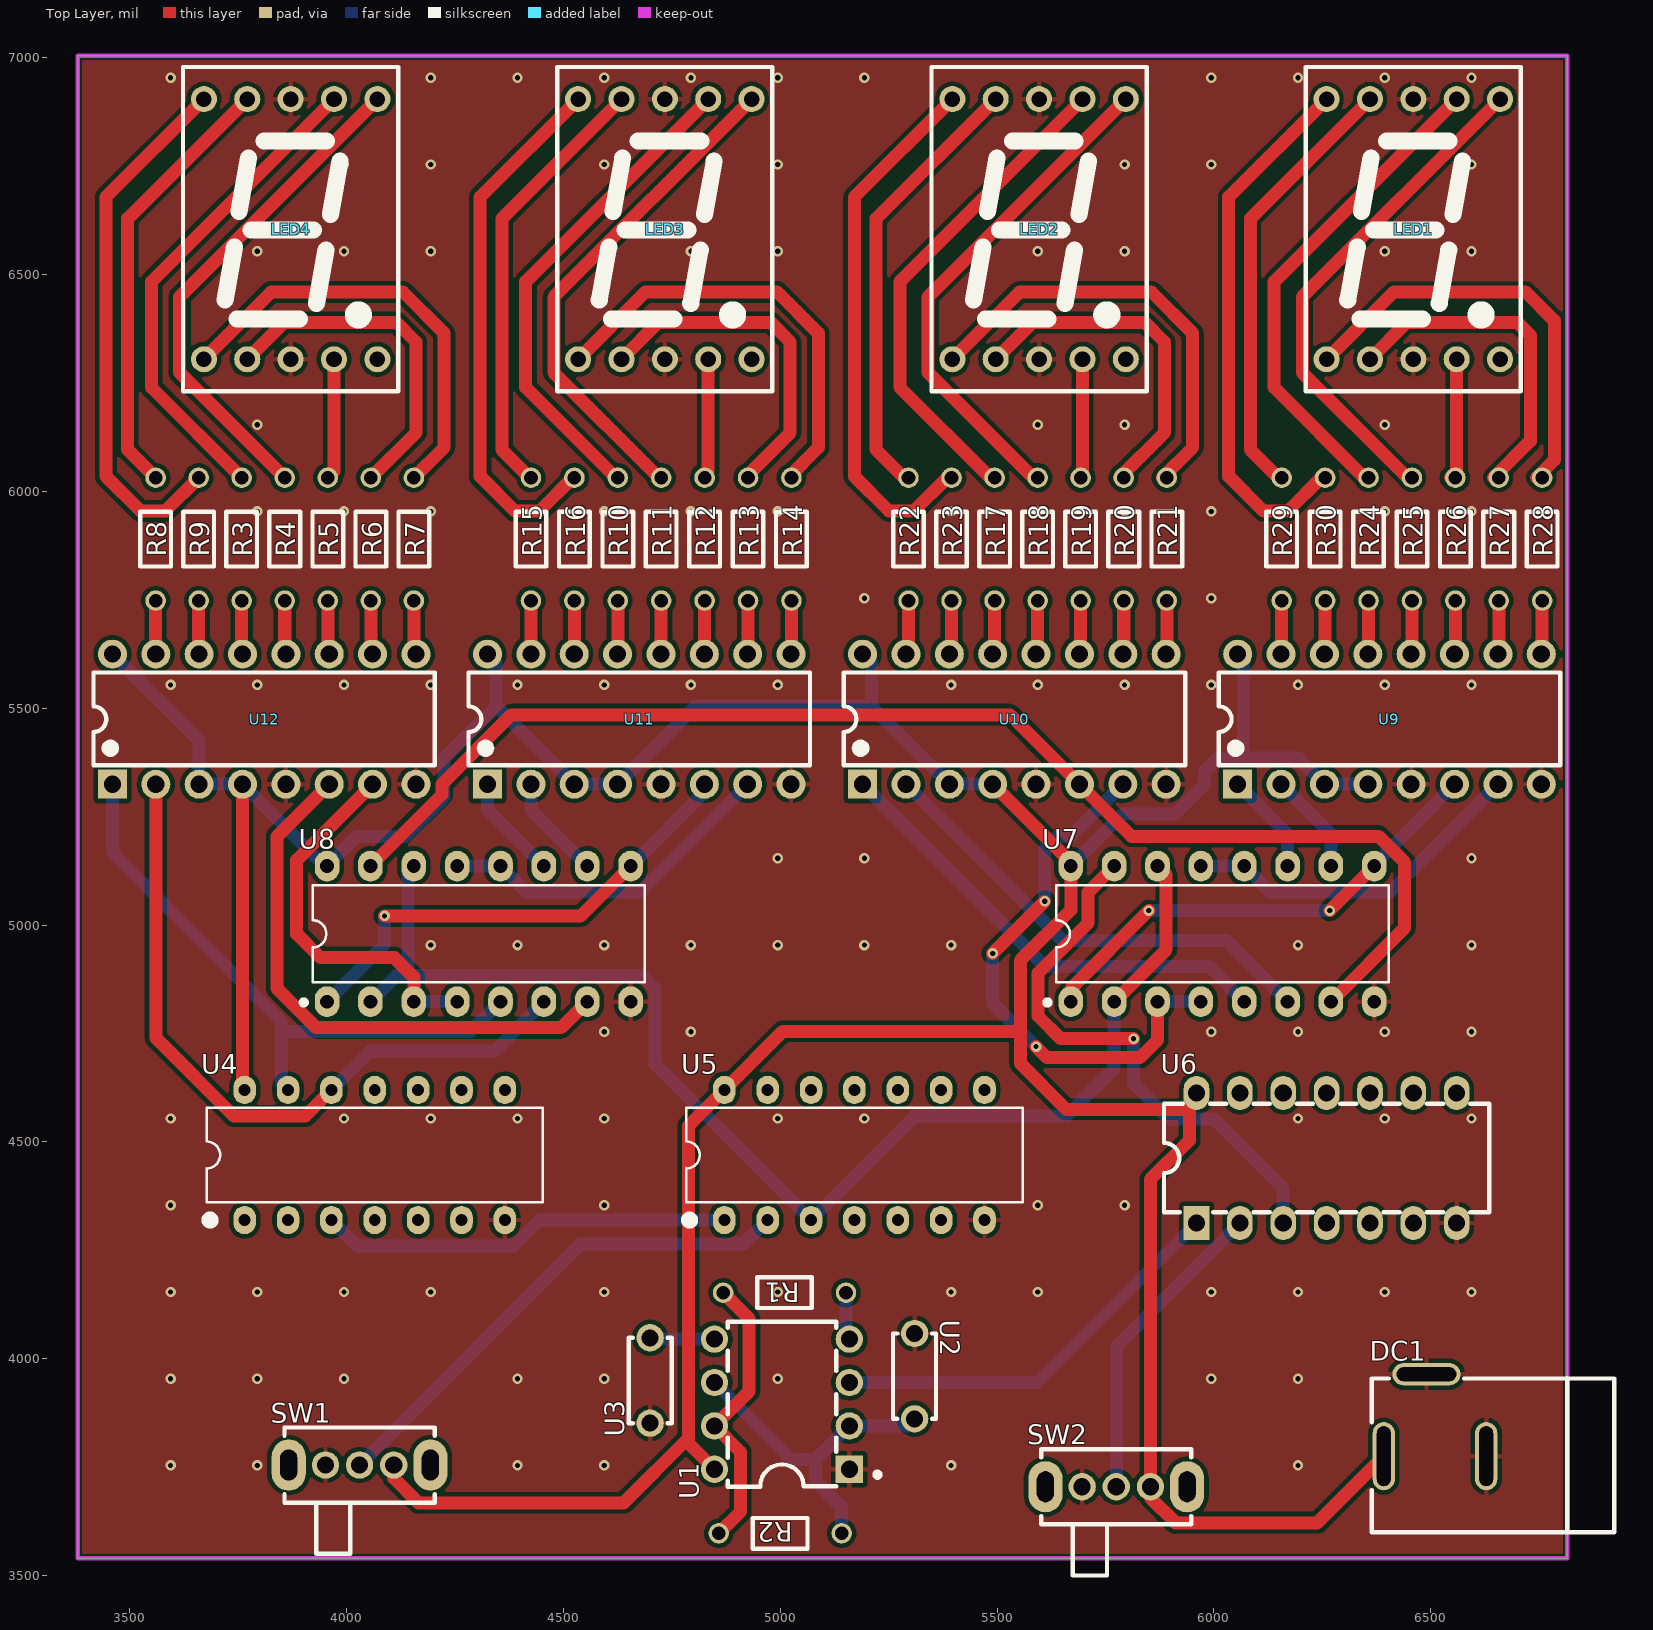
[diagram p0: Top Layer view]
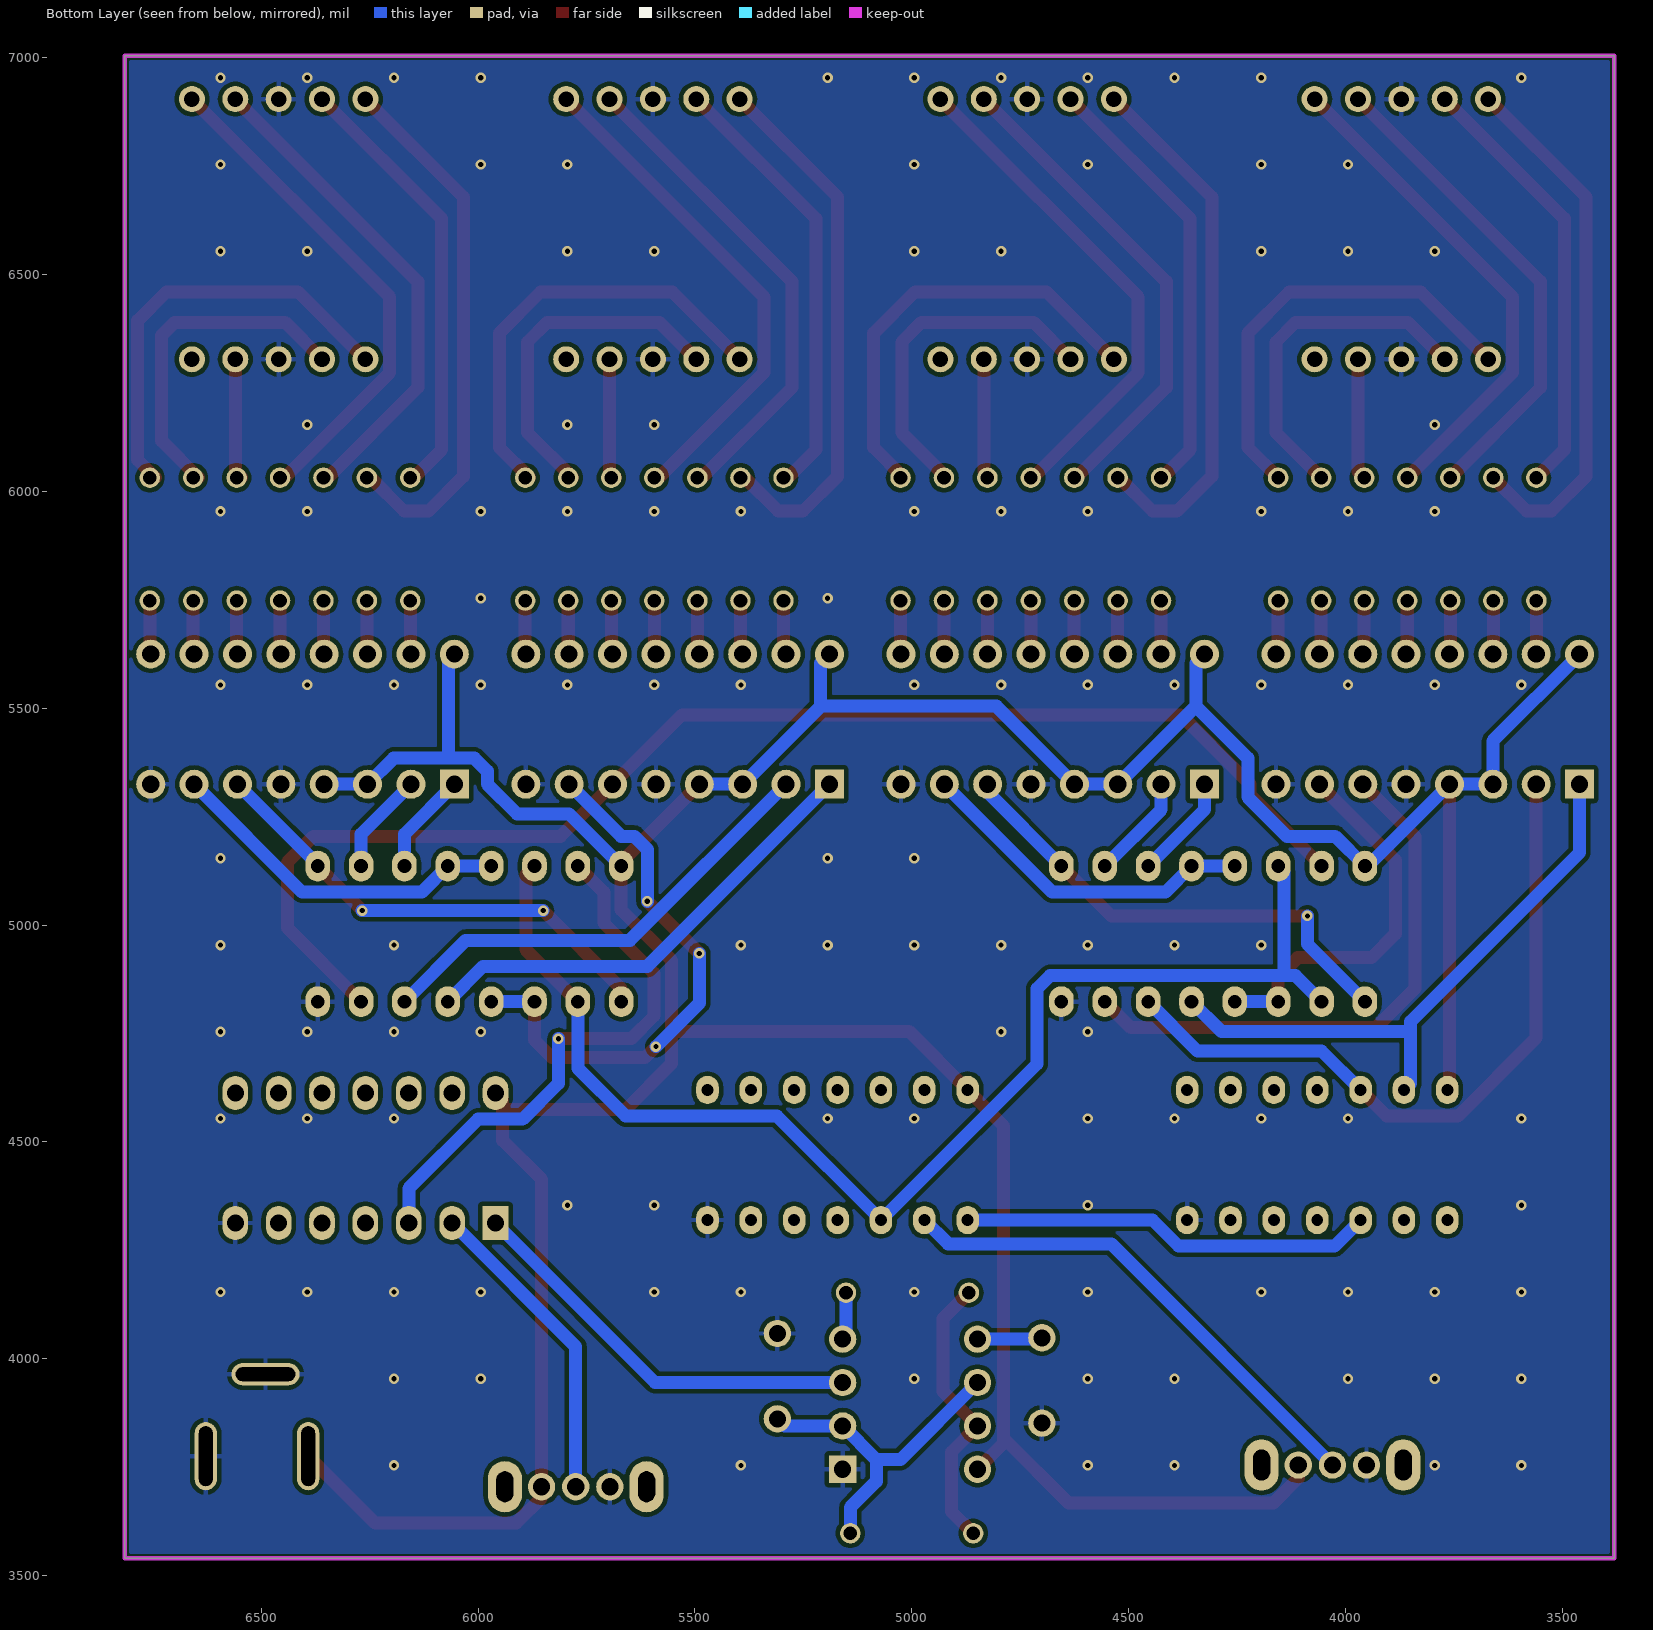
[diagram p1: Bottom Layer view, seen from below]
# Altium PCB MISC75414.pcbdoc
Units mil, origin at the board's own origin, x right, y up, seen from the top; angles counter-clockwise.
Board outline 3435 x 3465 mil, 2 copper layers (Top Layer, Bottom Layer), stack 62.206 mil thick; 49 components, 84 nets, 263 pads, 125 vias.

## Layer stack, top to bottom
Top Solder Mask Layer: solder mask 0.394, Dk 3.3
Top Layer: signal copper 1.379
Dielectric1: surface 59.449, FR4, Dk 4.5
Bottom Layer: signal copper 1.378
Bottom Solder Mask Layer: solder mask 0.394, Dk 3.3

## Board outline
3380,7005 3380,3540 6815,3540 6815,7005

## Design rules (kind name [scope] priority, off if disabled: settings)
BoardOutlineClearance copperThickness2oz_1 [All] p2 off: genericclearance=7.99 ignorepadtopadclearanceinfootprint=FALSE except(0: Arc-SplitContinuation Track-SplitContinuation SMDPad-SplitContinuation THPad-SplitContinuation Via-SplitContinuation Fill-SplitContinuation Region-SplitContinuation Poly-SplitContinuation Text-SplitContinuation Hole-SplitContinuation; 5.98: Arc-CutoutEdge SMDPad-CutoutEdge THPad-CutoutEdge Via-CutoutEdge Fill-CutoutEdge Region-CutoutEdge Text-CutoutEdge; 6.93: Hole-OutlineEdge Hole-CutoutEdge; 10: Poly-OutlineEdge Poly-CutoutEdge; 11.81: Arc-OutlineEdge Track-OutlineEdge SMDPad-OutlineEdge THPad-OutlineEdge Via-OutlineEdge Fill-OutlineEdge Region-OutlineEdge Text-OutlineEdge Track-CutoutEdge)
BoardOutlineClearance copperThickness1oz_1 [All] p4: genericclearance=4.02 ignorepadtopadclearanceinfootprint=FALSE except(0: Arc-SplitContinuation Track-SplitContinuation SMDPad-SplitContinuation THPad-SplitContinuation Via-SplitContinuation Fill-SplitContinuation Region-SplitContinuation Poly-SplitContinuation Text-SplitContinuation Hole-SplitContinuation; 6: SMDPad-CutoutEdge THPad-CutoutEdge Via-CutoutEdge Fill-CutoutEdge Region-CutoutEdge Text-CutoutEdge; 6.93: Hole-OutlineEdge Hole-CutoutEdge; 10: Poly-OutlineEdge Poly-CutoutEdge; 11.8: Arc-OutlineEdge Track-OutlineEdge SMDPad-OutlineEdge THPad-OutlineEdge Via-OutlineEdge Fill-OutlineEdge Region-OutlineEdge Text-OutlineEdge; 11.81: Arc-CutoutEdge Track-CutoutEdge)
Clearance copperThickness2oz [All] p1 off: gap=7.99 ignorepadtopadclearanceinfootprint=FALSE except(5.98: SMDPad-Track SMDPad-SMDPad THPad-Track SMDPad-THPad THPad-THPad Track-Via SMDPad-Via THPad-Via Via-Via Fill-Track Region-Track Fill-SMDPad Region-SMDPad Fill-THPad Region-THPad Fill-Via Region-Via Fill-Fill Fill-Region Region-Region Arc-Track Arc-SMDPad Arc-THPad Arc-Via Fill-Arc Region-Arc Arc-Arc Text-Track SMDPad-Text Text-THPad Text-Via Fill-Text Region-Text Arc-Text Text-Text; 6.93: Hole-Track Hole-SMDPad Hole-THPad Hole-Via Fill-Hole Region-Hole Hole-Arc Hole-Text; 10: Poly-Track Poly-SMDPad Poly-THPad Poly-Via Poly-Fill Poly-Region Poly-Poly Poly-Arc Poly-Text Poly-Hole)
Clearance copperThickness1oz [All] p3: gap=4.02 ignorepadtopadclearanceinfootprint=FALSE except(5.98: SMDPad-Track SMDPad-SMDPad THPad-Track SMDPad-THPad THPad-THPad Track-Via SMDPad-Via THPad-Via Via-Via Fill-Track Region-Track Fill-SMDPad Region-SMDPad Fill-THPad Region-THPad Fill-Via Region-Via Fill-Fill Fill-Region Region-Region; 6: Arc-Track Arc-SMDPad Arc-THPad Arc-Via Fill-Arc Region-Arc Arc-Arc Text-Track SMDPad-Text Text-THPad Text-Via Fill-Text Region-Text Arc-Text Text-Text; 6.93: Hole-Track Hole-SMDPad Hole-THPad Hole-Via Fill-Hole Region-Hole Hole-Arc Hole-Text; 10: Poly-Track Poly-SMDPad Poly-THPad Poly-Via Poly-Fill Poly-Region Poly-Poly Poly-Arc Poly-Text Poly-Hole)
Creepage creepage [All] p1: checkdistance=0 ignoreinternallayers=TRUE applytopolygonpour=TRUE
DiffPairsRouting differentialPair [All] p1: maxlimit=6 minlimit=6 mostfreqgap=6 toplayer_minwidth=5 toplayer_prefwidth=10 toplayer_maxwidth=100 toplayer_mingap=6 toplayer_prefgap=6 toplayer_maxgap=6 bottomlayer_minwidth=5 bottomlayer_prefwidth=10 bottomlayer_maxwidth=100 bottomlayer_mingap=6 bottomlayer_prefgap=6 bottomlayer_maxgap=6 maxuncoupledlength=10
HoleToHoleClearance otherClearance [All] p1: gap=11.81 allowstackedmicrovias=TRUE
Length netLength [All] p1: minlimit=0 maxlimit=0
MatchedLengths netLengthTolerance [All] p1: tolerance=1000
PasteMaskExpansion pasteMaskExpansion [All] p1: expansion=0
PlaneConnect innerPlane [All] p1: planeconnectstyle=Relief reliefexpansion=20 reliefentries=4 reliefconductorwidth=10 reliefairgap=10
PolygonConnect copperRegion [(InNet('GND'))] p1: connectstyle=Relief reliefconductorwidth=10 reliefentries=4 polygonreliefangle="90 Angle" airgapwidth=10 via.connectstyle=Relief via.reliefconductorwidth=10 via.reliefentries=4 via.polygonreliefangle="90 Angle" via.airgapwidth=10
RoutingVias viaSize [All] p1: holewidth=12.01 width=24.02 viastyle="Through Hole" minholewidth=11.81 minwidth=19.68 maxholewidth=248.03 maxwidth=393.7
SolderMaskExpansion solderMaskExpansion [IsVia] p1: expansion=-1000 istentingtop=TRUE
SolderMaskExpansion solderMaskExpansion [All] p2: expansion=2 istentingtop=FALSE
Width copperThickness2oz_2 [All] p1 off: maxlimit=100 minlimit=8 preferedwidth=10
Width copperThickness1oz_2 [All] p2: maxlimit=10 minlimit=10 preferedwidth=10 toplayer_minwidth=30 toplayer_maxwidth=100 toplayer_prefwidth=30 bottomlayer_minwidth=30 bottomlayer_maxwidth=100 bottomlayer_prefwidth=30

## Components (designator, comment, footprint, x,y, rotation, side; value= is the part's Value field where it differs from the comment)
DC1 "" DC-2.0 6515,3765 r0 top
LED1 "" LED-SEG-TH_10P-L12.6-W19.0-P2.54-S15.24-BL 6460,6605 r0 top
LED2 "" LED-SEG-TH_10P-L12.6-W19.0-P2.54-S15.24-BL 5596.99,6605 r0 top
LED3 "" LED-SEG-TH_10P-L12.6-W19.0-P2.54-S15.24-BL 4733.98,6605 r0 top
LED4 "" LED-SEG-TH_10P-L12.6-W19.0-P2.54-S15.24-BL 3870.96,6605 r0 top
R1 "68kΩ" Res_1/8W 5010,4150.05 r0 top
R2 "10kΩ" Res_1/8W 5000,3595.05 r0 top
R3 "300Ω" Res_1/8W 3760.62,5890.17 r90 top
R4 "300Ω" Res_1/8W 3859.89,5890.17 r90 top
R5 "300Ω" Res_1/8W 3959.16,5890.17 r90 top
R6 "300Ω" Res_1/8W 4058.43,5890.17 r90 top
R7 "300Ω" Res_1/8W 4157.7,5890.17 r90 top
R8 "300Ω" Res_1/8W 3562.08,5890.17 r90 top
R9 "300Ω" Res_1/8W 3661.35,5890.17 r90 top
R10 "300Ω" Res_1/8W 4627.91,5890.17 r90 top
R11 "300Ω" Res_1/8W 4728.02,5890.17 r90 top
R12 "300Ω" Res_1/8W 4828.12,5890.17 r90 top
R13 "300Ω" Res_1/8W 4928.23,5890.17 r90 top
R14 "300Ω" Res_1/8W 5028.33,5890.17 r90 top
R15 "300Ω" Res_1/8W 4427.7,5890.17 r90 top
R16 "300Ω" Res_1/8W 4527.81,5890.17 r90 top
R17 "300Ω" Res_1/8W 5496.87,5890.17 r90 top
R18 "300Ω" Res_1/8W 5596.14,5890.17 r90 top
R19 "300Ω" Res_1/8W 5695.42,5890.17 r90 top
R20 "300Ω" Res_1/8W 5794.69,5890.17 r90 top
R21 "300Ω" Res_1/8W 5893.96,5890.17 r90 top
R22 "300Ω" Res_1/8W 5298.33,5890.17 r90 top
R23 "300Ω" Res_1/8W 5397.6,5890.17 r90 top
R24 "300Ω" Res_1/8W 6359.17,5890.17 r90 top
R25 "300Ω" Res_1/8W 6459.27,5890.17 r90 top
R26 "300Ω" Res_1/8W 6559.38,5890.17 r90 top
R27 "300Ω" Res_1/8W 6659.48,5890.17 r90 top
R28 "300Ω" Res_1/8W 6759.58,5890.17 r90 top
R29 "300Ω" Res_1/8W 6158.96,5890.17 r90 top
R30 "300Ω" Res_1/8W 6259.06,5890.17 r90 top
SW1 "" 拨动开关_侧 4030,3755 r0 top
SW2 "" 拨动开关_侧 5775,3705 r0 top
U1 "NE555PE4" PDIP-8_L9.6-W6.4-P2.54-LS7.9-BL-1 5003.9,3895.25 r90 top
U2 "100nF" CAP-TH_L5.0-W2.5-P5.00-D1.0 5310,3960.05 r270 top
U3 "10nF" CAP-TH_L5.0-W2.5-P5.00-D1.0 4700,3950.05 r90 top
U4 "NTE74LS08" DIP-14_L19.6-W6.4-P2.54-LS7.6-BL 4065,4470 r0 top
U5 "NTE74LS32" DIP-14_L19.6-W6.4-P2.54-LS7.6-BL 5171.1,4470 r0 top
U6 "SN74LS00N(XBLW)" PDIP-14_L19.3-W6.4-P2.54-LS7.6-BL 6260,4463.11 r0 top
U7 "SN74LS390NE4" PDIP-16_L19.3-W6.4-P2.54-LS7.94-BL 6020,4980 r0 top
U8 "SN74LS390NE4" PDIP-16_L19.3-W6.4-P2.54-LS7.94-BL 4305,4980 r0 top
U9 "CD74HC4511E" PDIP-16_L19.7-W6.6-P2.54-LS7.6-BL 6405,5475 r0 top
U10 "CD74HC4511E" PDIP-16_L19.7-W6.6-P2.54-LS7.6-BL 5540,5475 r0 top
U11 "CD74HC4511E" PDIP-16_L19.7-W6.6-P2.54-LS7.6-BL 4675,5475 r0 top
U12 "CD74HC4511E" PDIP-16_L19.7-W6.6-P2.54-LS7.6-BL 3810,5475 r0 top

## Footprints (in the part's own frame and the unit in brackets; to place one, negate y for a bottom-side part, rotate by r counter-clockwise, add the part's x,y. Pads: shape width x height; smd on the part's side, far side on the other; paste and mask are expansions set on the pad)
CAP-TH_L5.0-W2.5-P5.00-D1.0 [mm]
  round 1.6 hole 1: 1(-2.5,0) 2(2.5,0)
  silkscreen extent -2.5,-1.27 2.5,1.25
DC-2.0 [mil]
  oval 157.5x51.2 hole 31.5 slot 137.8 at 0 deg paste+0 mask+2: 2(-24.7,199.5)
  oval 51.2x157.5 hole 31.5 slot 137.8 at 90 deg paste+0 mask+2: 3(113.1,10.5) 4(-123.1,10.5)
  silkscreen extent -151,-165 408,190
DIP-14_L19.6-W6.4-P2.54-LS7.6-BL [mm]
  oval 1.32x1.65 hole 0.7: 1(-7.62,-3.81) 2(-5.08,-3.81) 3(-2.54,-3.81) 4(0,-3.81) 5(2.54,-3.81) 6(5.08,-3.81) 7(7.62,-3.81) 8(7.62,3.81) 9(5.08,3.81) 10(2.54,3.81) 11(0,3.81) 12(-2.54,3.81) 13(-5.08,3.81) 14(-7.62,3.81)
  silkscreen extent -9.85,-4.01 9.85,2.76
LED-SEG-TH_10P-L12.6-W19.0-P2.54-S15.24-BL [mil]
  round 60 hole 36: 1(-200,-300) 2(-100,-300) 3(0,-300) 4(100,-300) 5(200,-300) 6(200,300) 7(100,300) 8(0,300) 9(-100,300) 10(-200,300)
  silkscreen extent -248,-374 248,374
PDIP-8_L9.6-W6.4-P2.54-LS7.9-BL-1 [mil]
  rect 63x63 hole 39.37: 1(-150,-155.51)
  round 63 hole 39.37: 2(-50,-155.51) 3(50,-155.51) 4(150,-155.51) 5(150,155.52) 6(50,155.52) 7(-50,155.52) 8(-150,155.52)
  silkscreen extent -190,-226 190,125
PDIP-14_L19.3-W6.4-P2.54-LS7.6-BL [mm]
  rect 1.5x2 hole 1: 1(-7.62,-3.81)
  oval 1.5x2 hole 1: 2(-5.08,-3.81) 3(-2.54,-3.81) 4(0,-3.81) 5(2.54,-3.81) 6(5.08,-3.81) 7(7.62,-3.81) 8(7.62,3.81) 9(5.08,3.81) 10(2.54,3.81) 11(0,3.81) 12(-2.54,3.81) 13(-5.08,3.81) 14(-7.62,3.81)
  silkscreen extent -9.53,-3.17 9.53,3.17
PDIP-16_L19.3-W6.4-P2.54-LS7.94-BL [mm]
  oval 1.44x1.8 hole 0.8: 1(-8.89,-3.97) 2(-6.35,-3.97) 3(-3.81,-3.97) 4(-1.27,-3.97) 5(1.27,-3.97) 6(3.81,-3.97) 7(6.35,-3.97) 8(8.89,-3.97) 9(8.89,3.97) 10(6.35,3.97) 11(3.81,3.97) 12(1.27,3.97) 13(-1.27,3.97) 14(-3.81,3.97) 15(-6.35,3.97) 16(-8.89,3.97)
  silkscreen extent -10.41,-4.17 9.73,2.84
PDIP-16_L19.7-W6.6-P2.54-LS7.6-BL [mm]
  rect 1.7x1.7 hole 1: 1(-8.89,-3.81)
  round 1.7 hole 1: 2(-6.35,-3.81) 3(-3.81,-3.81) 4(-1.27,-3.81) 5(1.27,-3.81) 6(3.81,-3.81) 7(6.35,-3.81) 8(8.89,-3.81) 9(8.89,3.81) 10(6.35,3.81) 11(3.81,3.81) 12(1.27,3.81) 13(-1.27,3.81) 14(-3.81,3.81) 15(-6.35,3.81) 16(-8.89,3.81)
  silkscreen extent -10,-2.7 10,2.73
Res_1/8W [mil]
  round 47.2 hole 31.5 paste+0 mask+2: 1(-141.7,2.48) 2(141.7,2.48)
  silkscreen extent -63,-33 63,38
拨动开关_侧 [mil]
  round 63 hole 39.4 paste+0 mask+2: 1(-78.7,0) 2(0,0) 3(78.7,0)
  oval 78.7x118.1 hole 39.4 slot 70.9 at 90 deg paste+0 mask+2: 4(163.4,0) 5(-163.4,0)
  silkscreen extent -173,-205 173,87

## Via types
v1: diameter 24.02, hole 12, Top Layer to Bottom Layer, 125 vias

## Nets (pads, with @x,y where several pads share a name; then routed paths per layer and width w, separated by ;. In a path a pad name is that pad's centre, name@x,y a point inside that pad or via, vN(x,y) a via of type N, cw(c..) or ccw(c..) an arc to the next point about the centre after c; other vN are vias at no path point)
$1N1: R1.2 U1.4 | length 110.5
  Bottom Layer w30: R1.2 5151.7,4052.96 U1.4
$1N2: R1.1 R2.1 U1.7 | length 658.6
  Top Layer w30: R2.1 4908.39,3647.61 4908.39,3785.25 U1.7 4928.3,3925.17 4928.3,4092.52 R1.1
$1N3: R2.2 U1.2 U1.6 U2.2 | length 769.1
  Bottom Layer w30: U1.6 5026.09,3767.55 5081.7,3767.55 ; R2.2 5141.7,3657.52 5081.7,3717.52 5081.7,3767.55 ; U2.2 5293.63,3845.25 U1.2 5081.7,3767.55
$1N6: U1.5 U3.2 | length 149.7
  Bottom Layer w30: U3.2 4703.22,4045.25 U1.5
$1N9: SW1.2 U5.2 | length 1175.1
  Bottom Layer w30: SW1.2 4540,4265 4916.1,4265 U5.2
$1N10: U4.3 U5.1 | length 955.8
  Bottom Layer w30: U4.3 4025,4260 4385,4260 4445,4320 U5.1
$1N17: U1.3 U6.1 | length 953
  Bottom Layer w30: U1.3 5592.14,3945.25 U6.1
$1N18: SW2.2 U6.2 | length 726.2
  Bottom Layer w30: SW2.2 5775,4028.11 U6.2
$1N21: U6.3 U7.15 | length 1289.1
  Top Layer w30: U7.15 5710,5076.3 5710,5005 5594.32,4889.32 5594.32,4790.68 5646.89,4738.11 v1(5815,4738.11)
  Bottom Layer w30: v1(5815,4738.11) 5815,4635 5897.24,4552.76 6000.36,4552.76 6160,4393.11 U6.3
$1N24: U5.3 U7.2 U7.14 U8.2 U8.14 | length 3002.7
  Top Layer w30: U7.2 5890,4943.7 5890,5116.3 U7.14
  Bottom Layer w30: U8.2 4115,4883.7 4141.1,4883.7 ; U8.14 4141.1,5122.4 4141.1,4883.7 ; U7.2 5770,4670 5660,4560 5311.1,4560 U5.3 4711.1,4680 4711.1,4853.7 4681.1,4883.7 4141.1,4883.7
$1N39: U7.1 U7.9 U9.6 | length 1112.4
  Top Layer w30: U7.1 5670,4853.7 v1(5850,5033.7) ; v1(6267.4,5033.7) U7.9
  Bottom Layer w30: v1(5850,5033.7) v1(6267.4,5033.7) ; U7.9 6370,5140 U9.6
$1N40: U7.10 U9.2 | length 236.3
  Bottom Layer w30: U9.2 6270,5210 U7.10
$1N41: U7.11 U9.1 | length 236.3
  Bottom Layer w30: U9.1 6170,5210 U7.11
$1N42: U7.12 U7.13 U9.7 | length 812.9
  Bottom Layer w30: U7.13 U7.12 6130,5076.3 6406.3,5076.3 U9.7
$1N53: U7.3 U7.4 U10.7 | length 1283.9
  Top Layer w30: v1(5490,4935) v1(5610,5055) ; v1(5590,4720) 5615,4695 5830,4695 5870,4735 U7.3
  Bottom Layer w30: v1(5490,4935) 5490,4820 v1(5590,4720) ; v1(5610,5055) 5610,5175 5640,5205 5670,5205 U10.7 ; U7.3 U7.4
$1N54: U7.5 U10.1 | length 1087.6
  Bottom Layer w30: U10.1 5610,4905 5988.7,4905 U7.5
$1N55: U7.6 U10.2 | length 1087.6
  Bottom Layer w30: U10.2 5650,4965 6028.7,4965 U7.6
$1N56: U7.7 U8.15 U10.6 | length 3075.9
  Top Layer w30: U8.15 4220,5301.3 4220,5325 4380.01,5485 5530,5485 U10.6 5810,5205 6380,5205 6440,5145 6440,4993.7 U7.7
$1N67: U8.12 U8.13 U11.7 | length 797.9
  Bottom Layer w30: U8.13 U8.12 4415,5076.3 4676.3,5076.3 U11.7
$1N68: U8.11 U11.1 | length 242.5
  Bottom Layer w30: U11.1 4325,5266.3 U8.11
$1N69: U8.10 U11.2 | length 242.5
  Bottom Layer w30: U11.2 4425,5266.3 U8.10
$1N70: U8.1 U8.9 U11.6 | length 1126.7
  Top Layer w30: v1(4087.6,5021.3) 4540,5021.3 U8.9
  Bottom Layer w30: U8.1 4087.6,4956.3 v1(4087.6,5021.3) ; U8.9 4825,5306.3 U11.6
$1N81: U8.3 U8.4 U12.7 | length 885.2
  Top Layer w30: U12.7 3885,5150 3885,5131.64 3885,4980 3940,4925 4110,4925 4155,4880 U8.3
  Bottom Layer w30: U8.3 U8.4
$1N82: U4.13 U8.5 U12.1 | length 1406.2
  Bottom Layer w30: U12.1 3460,5167.52 3850,4777.52 3850,4755 ; U4.13 3850,4635 3850,4755 ; U8.5 4286.3,4755 3850,4755
$1N83: U4.12 U8.6 U12.2 | length 1663.8
  Top Layer w30: U12.2 3560,4740 3740,4560 3905,4560 U4.12
  Bottom Layer w30: U4.12 4055,4710 4341.3,4710 U8.6
$1N84: U8.7 U12.6 | length 1298.1
  Top Layer w30: U12.6 3840,5205 3840,4853.7 3930,4763.7 4495,4763.7 U8.7
$1N94: R3.1 U12.13 | length 123.5
  Top Layer w30: U12.13@3758.14,5625 R3.1
$1N95: LED4.7 R3.2 | length 1133.7
  Top Layer w30: R3.2 3550,6240.01 3550,6484.04 LED4.7
$1N96: R4.1 U12.12 | length 123.5
  Top Layer w30: U12.12@3857.41,5625 R4.1
$1N97: LED4.6 R4.2 | length 1162.4
  Top Layer w30: R4.2 3615,6274.29 3615,6449.04 LED4.6
$1N98: R5.1 U12.11 | length 123.5
  Top Layer w30: U12.11@3956.68,5625 R5.1
$1N99: LED4.4 R5.2 | length 279
  Top Layer w30: R5.2 3970.96,6046.15 LED4.4
$1N100: R6.1 U12.10 | length 123.5
  Top Layer w30: U12.10@4055.95,5625 R6.1
$1N101: LED4.2 R6.2 | length 799.1
  Top Layer w30: LED4.2 3855.96,6390 4115,6390 4160,6345 4160,6135.92 R6.2
$1N102: R7.1 U12.9 | length 123.5
  Top Layer w30: U12.9@4155.22,5625 R7.1
$1N103: LED4.1 R7.2 | length 1019.6
  Top Layer w30: LED4.1 3825.96,6460 4130,6460 4225,6365 4225,6101.65 R7.2
$1N104: R8.1 U12.15 | length 123.5
  Top Layer w30: U12.15@3559.6,5625 R8.1
$1N105: LED4.9 R8.2 | length 1014.2
  Top Layer w30: R8.2 3495,6096.47 3495,6629.04 LED4.9
$1N106: R9.1 U12.14 | length 123.5
  Top Layer w30: U12.14@3658.87,5625 R9.1
$1N107: LED4.10 R9.2 | length 1242.4
  Top Layer w30: R9.2 3582,5955 3525,5955 3445,6035 3445,6679.04 LED4.10
$1N108: R16.1 U11.14 | length 123.5
  Top Layer w30: U11.14@4525.33,5625 R16.1
$1N109: LED3.10 R16.2 | length 1242.4
  Top Layer w30: R16.2@4521.88,6031.87 4445.01,5955 4388.01,5955 4308.01,6035 4308.01,6679.04 LED3.10
$1N110: R15.1 U11.15 | length 123.5
  Top Layer w30: U11.15@4425.23,5625 R15.1
$1N111: LED3.9 R15.2 | length 1014.2
  Top Layer w30: R15.2@4422.61,6031.87 4358.01,6096.47 4358.01,6629.04 LED3.9
$1N112: R14.1 U11.9 | length 123.5
  Top Layer w30: U11.9@5025.85,5625 R14.1
$1N113: LED3.1 R14.2 | length 1019.6
  Top Layer w30: LED3.1 4688.98,6460 4993.01,6460 5088.01,6365 5088.01,6101.65 R14.2@5018.24,6031.87
$1N114: R13.1 U11.10 | length 123.5
  Top Layer w30: U11.10@4925.75,5625 R13.1
$1N115: LED3.2 R13.2 | length 799.1
  Top Layer w30: LED3.2 4718.98,6390 4978.01,6390 5023.01,6345 5023.01,6135.92 R13.2@4918.97,6031.87
$1N116: R12.1 U11.11 | length 123.5
  Top Layer w30: U11.11@4825.64,5625 R12.1
$1N117: LED3.4 R12.2 | length 279
  Top Layer w30: R12.2@4819.7,6031.87 4833.98,6046.15 LED3.4
$1N118: R11.1 U11.12 | length 123.5
  Top Layer w30: U11.12@4725.54,5625 R11.1
$1N119: LED3.6 R11.2 | length 1162.4
  Top Layer w30: R11.2@4720.42,6031.87 4478.01,6274.29 4478.01,6449.04 LED3.6
$1N120: R10.1 U11.13 | length 123.5
  Top Layer w30: U11.13@4625.44,5625 R10.1
$1N121: LED3.7 R10.2 | length 1133.7
  Top Layer w30: R10.2@4621.15,6031.87 4413.01,6240.01 4413.01,6484.04 LED3.7
$1N122: R23.1 U10.14 | length 123.5
  Top Layer w30: U10.14@5395.13,5625 R23.1
$1N123: LED2.10 R23.2 | length 1242.4
  Top Layer w30: R23.2@5384.9,6031.87 5308.02,5955 5251.02,5955 5171.02,6035 5171.02,6679.04 LED2.10
$1N124: R22.1 U10.15 | length 123.5
  Top Layer w30: U10.15@5295.86,5625 R22.1
$1N125: LED2.9 R22.2 | length 1014.2
  Top Layer w30: R22.2@5285.62,6031.87 5221.02,6096.47 5221.02,6629.04 LED2.9
$1N126: R21.1 U10.9 | length 123.5
  Top Layer w30: U10.9@5891.48,5625 R21.1
$1N127: LED2.1 R21.2 | length 1019.6
  Top Layer w30: LED2.1 5551.99,6460 5856.02,6460 5951.02,6365 5951.02,6101.65 R21.2@5881.25,6031.87
$1N128: R20.1 U10.10 | length 123.5
  Top Layer w30: U10.10@5792.21,5625 R20.1
$1N129: LED2.2 R20.2 | length 799.1
  Top Layer w30: LED2.2 5581.99,6390 5841.02,6390 5886.02,6345 5886.02,6135.92 R20.2@5781.98,6031.87
$1N130: R19.1 U10.11 | length 123.5
  Top Layer w30: U10.11@5692.94,5625 R19.1
$1N131: LED2.4 R19.2 | length 279
  Top Layer w30: R19.2@5682.71,6031.87 5696.99,6046.15 LED2.4
$1N132: R18.1 U10.12 | length 123.5
  Top Layer w30: U10.12@5593.67,5625 R18.1
$1N133: LED2.6 R18.2 | length 1162.4
  Top Layer w30: R18.2@5583.44,6031.87 5341.02,6274.29 5341.02,6449.04 LED2.6
$1N134: R17.1 U10.13 | length 123.5
  Top Layer w30: U10.13@5494.4,5625 R17.1
$1N135: LED2.7 R17.2 | length 1133.7
  Top Layer w30: R17.2@5484.17,6031.87 5276.02,6240.01 5276.02,6484.04 LED2.7
$1N136: LED1.7 R24.2 | length 1133.7
  Top Layer w30: R24.2@6347.18,6031.87 6139.04,6240.01 6139.04,6484.04 LED1.7
$1N137: R24.1 U9.13 | length 123.5
  Top Layer w30: U9.13@6356.69,5625 R24.1
$1N138: R25.1 U9.12 | length 123.5
  Top Layer w30: U9.12@6456.8,5625 R25.1
$1N139: LED1.6 R25.2 | length 1162.4
  Top Layer w30: R25.2@6446.45,6031.87 6204.04,6274.29 6204.04,6449.04 LED1.6
$1N140: LED1.4 R26.2 | length 279
  Top Layer w30: R26.2@6545.72,6031.87 6560,6046.15 LED1.4
$1N141: R26.1 U9.11 | length 123.5
  Top Layer w30: U9.11@6556.9,5625 R26.1
$1N142: R27.1 U9.10 | length 123.5
  Top Layer w30: U9.10@6657,5625 R27.1
$1N143: LED1.2 R27.2 | length 781
  Top Layer w30: LED1.2 6445,6390 6700,6390 6730,6360 6730,6116.88 R27.2@6644.99,6031.87
$1N144: LED1.1 R28.2 | length 995.6
  Top Layer w30: LED1.1 6415,6460 6719.04,6460 6785,6394.04 6785,6072.61 R28.2@6744.26,6031.87
$1N145: R28.1 U9.9 | length 123.5
  Top Layer w30: U9.9@6757.11,5625 R28.1
$1N146: R29.1 U9.15 | length 123.5
  Top Layer w30: U9.15@6156.48,5625 R29.1
$1N147: LED1.9 R29.2 | length 1014.2
  Top Layer w30: R29.2@6148.64,6031.87 6084.04,6096.47 6084.04,6629.04 LED1.9
$1N148: LED1.10 R30.2 | length 1242.4
  Top Layer w30: R30.2@6247.91,6031.87 6171.03,5955 6114.04,5955 6034.04,6035 6034.04,6679.04 LED1.10
$1N149: R30.1 U9.14 | length 123.5
  Top Layer w30: U9.14@6256.59,5625 R30.1
GND: DC1.2 DC1.3 LED1.3 LED1.8 LED2.3 LED2.8 LED3.3 LED3.8 LED4.3 LED4.8 SW1.1 SW2.1 U1.1 U2.1 U3.1 U4.7 U5.7 U6.7 U7.8 U8.8 U9.5 U9.8 U10.5 U10.8 U11.5 U11.8 U12.5 U12.8
  other v1: 3594.1,3754.1 3794.1,3754.1 4394.1,3754.1 4594.1,3754.1 5394.1,3754.1 6194.1,3754.1 3594.1,3954.1 3794.1,3954.1 3994.1,3954.1 4394.1,3954.1 4594.1,3954.1 4994.1,3954.1 5994.1,3954.1 6194.1,3954.1 3594.1,4154.1 3794.1,4154.1 3994.1,4154.1 4194.1,4154.1 4594.1,4154.1 4994.1,4154.1 5394.1,4154.1 5594.1,4154.1 5994.1,4154.1 6194.1,4154.1 6394.1,4154.1 6594.1,4154.1 3594.1,4354.1 4594.1,4354.1 5594.1,4354.1 5794.1,4354.1 3594.1,4554.1 3994.1,4554.1 4194.1,4554.1 4394.1,4554.1 4594.1,4554.1 4994.1,4554.1 5194.1,4554.1 6194.1,4554.1 6394.1,4554.1 6594.1,4554.1 4594.1,4754.1 4794.1,4754.1 5994.1,4754.1 6194.1,4754.1 6394.1,4754.1 6594.1,4754.1 4194.1,4954.1 4394.1,4954.1 4594.1,4954.1 4794.1,4954.1 4994.1,4954.1 5194.1,4954.1 5394.1,4954.1 6194.1,4954.1 6594.1,4954.1 4994.1,5154.1 5194.1,5154.1 6594.1,5154.1 3594.1,5554.1 3794.1,5554.1 3994.1,5554.1 4194.1,5554.1 4394.1,5554.1 4594.1,5554.1 4794.1,5554.1 4994.1,5554.1 5394.1,5554.1 5594.1,5554.1 5794.1,5554.1 5994.1,5554.1 6194.1,5554.1 6394.1,5554.1 6594.1,5554.1 5194.1,5754.1 5994.1,5754.1 3794.1,5954.1 3994.1,5954.1 4194.1,5954.1 4594.1,5954.1 4794.1,5954.1 4994.1,5954.1 5394.1,5954.1 5594.1,5954.1 5794.1,5954.1 5994.1,5954.1 6394.1,5954.1 6594.1,5954.1 3794.1,6154.1 5594.1,6154.1 5794.1,6154.1 6394.1,6154.1 3794.1,6554.1 3994.1,6554.1 4194.1,6554.1 4794.1,6554.1 4994.1,6554.1 5594.1,6554.1 5794.1,6554.1 6394.1,6554.1 6594.1,6554.1 3994.1,6754.1 4194.1,6754.1 4594.1,6754.1 4994.1,6754.1 5794.1,6754.1 5994.1,6754.1 6594.1,6754.1 3594.1,6954.1 4194.1,6954.1 4394.1,6954.1 4594.1,6954.1 4794.1,6954.1 4994.1,6954.1 5194.1,6954.1 5994.1,6954.1 6194.1,6954.1 6394.1,6954.1 6594.1,6954.1
VCC: DC1.4 SW1.3 SW2.3 U1.8 U4.14 U5.14 U6.14 U7.16 U8.16 U9.3 U9.4 U9.16 U10.3 U10.4 U10.16 U11.3 U11.4 U11.16 U12.3 U12.4 U12.16 | length 10031.6
  Top Layer w30: U12.4 3760,4625 U4.14 ; SW1.3 4108.7,3725 4166.42,3667.29 4638.39,3667.29 4788.39,3817.29 ; U1.8 4788.39,3805.25 4788.39,3817.29 ; U10.4 5670,5145 U7.16 5670,5035 5553.7,4918.7 5553.7,4755 ; U6.14 5943.7,4596.81 5943.7,4575 ; DC1.4 6238.15,3621.75 5911.9,3621.75 5853.7,3679.95 SW2.3 5853.7,4413.74 5943.7,4503.74 5943.7,4575 ; 4788.39,3817.29 4788.39,4537.28 U5.14 5006.1,4755 5553.7,4755 ; 5553.7,4755 5553.7,4681.3 5660,4575 5943.7,4575
  Bottom Layer w30: U12.16 3660,5425 U12.3 U12.4 3948.7,5136.3 U8.16 4023.7,5205 4135,5205 4225,5295 4225,5385 4345,5505 ; U11.16 4345,5605 4345,5505 ; U10.16 5210,5605 5210,5505 ; U10.4 U10.3 5210,5505 ; U7.16 5790,5256.3 5910,5256.3 5978.7,5325 5978.7,5355 6008.7,5385 6068.7,5385 ; U9.16 6068.7,5611.3 6068.7,5385 ; U9.4 U9.3 6195,5385 6068.7,5385 ; 4345,5505 U11.3 U11.4 4805,5505 5210,5505
pads on no net: LED1.5 LED2.5 LED3.5 LED4.5 SW1.4 SW1.5 SW2.4 SW2.5 U4.1 U4.2 U4.4 U4.5 U4.6 U4.8 U4.9 U4.10 U4.11 U5.4 U5.5 U5.6 U5.8 U5.9 U5.10 U5.11 U5.12 U5.13 U6.4 U6.5 U6.6 U6.8 U6.9 U6.10 U6.11 U6.12 U6.13

## Polygon pours and split planes (outlines as drawn)
GND on Top Layer (solid, remove dead copper, pour order 0): 3000,7050 3000,3000 7285,3000 7285,7050
GND on Bottom Layer (solid, remove dead copper, pour order 2): 3235,7185 3235,3080 7195,3080 7195,7185

## Keep-outs
Board Outline Layer:
  the board outline again, w10